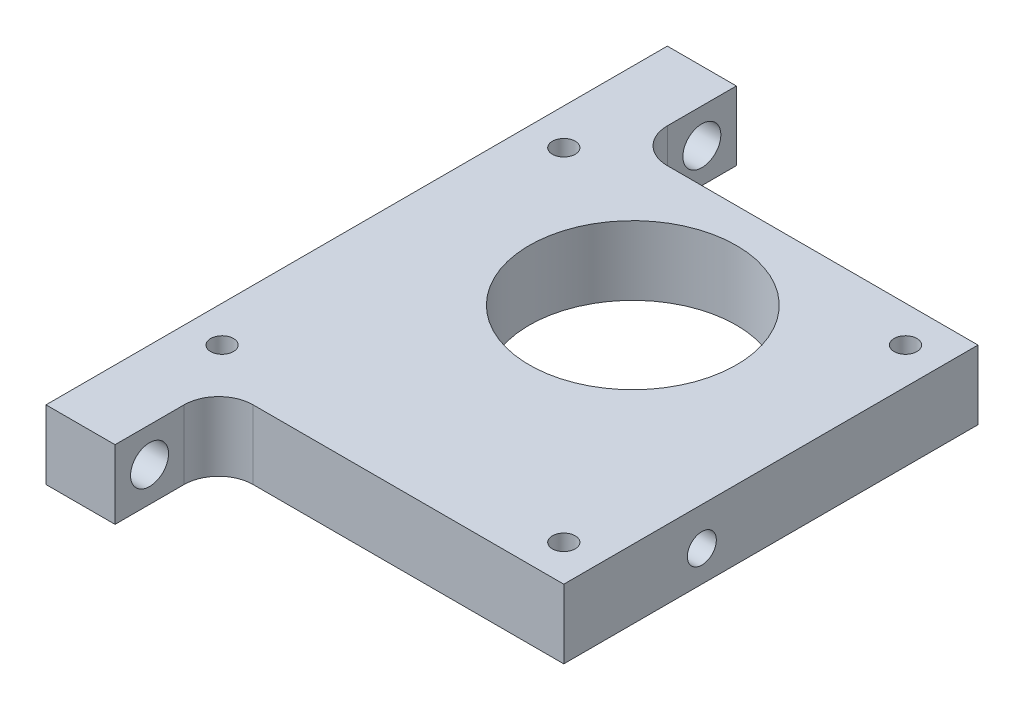
SolidWorks part; units mm, degrees
ref_plane "Front Plane" through (0, 0, 0) normal (0, 0, 1) x (1, 0, 0)
ref_plane "Top Plane" through (0, 0, 0) normal (0, 1, 0) x (1, 0, 0)
ref_plane "Right Plane" through (0, 0, 0) normal (1, 0, 0) x (0, 0, -1)
sketch "Sketch1" plane through (0, 0, 0) normal (0, 1, 0) x (1, 0, 0)
  line L1 (30, -45) -> (-30, -45)
  line L2 (30, -45) -> (30, 45)
  line L3 (30, 45) -> (-30, 45)
  line L4 (-30, -45) -> (-30, 45)
  line L5 (30, -45) -> (-30, 45) construction
  line L6 (30, 45) -> (-30, -45) construction
  point P0 (0, 0)
  dimension "D1" = 90
  dimension "D2" = 60
extrude "Boss-Extrude1" add sketch "Sketch1" along normal blind 10
sketch "Sketch4" plane through (0, 0, 0) normal (0, -1, 0) x (1, 0, 0)
  line L1 (0, 0) -> (0, -10) construction
  line L2 (30, -45) -> (-30, -45) construction
  circle A0 centre (0, -10) radius 15
  dimension "D1" = 35
  dimension "D2" = 30
extrude "Cut-Extrude3" cut sketch "Sketch4" against normal through all
hole_wizard "M4 Tapped Hole1" positions "Sketch6" profile "Sketch5" tap size "M4" standard "GB" end condition through all
sketch "Sketch6" plane through (0, 0, 0) normal (0, 1, 0) x (1, 0, 0)
  line L0 (-24.7487, -24.7475) -> (24.7487, -24.7475) construction
  line L1 (24.7487, -24.7475) -> (24.7487, 24.75) construction
  line L2 (24.7487, 24.75) -> (-24.7487, 24.75) construction
  line L3 (-24.7487, 24.75) -> (-24.7487, -24.7475) construction
  line L5 (0, 10) -> (0, 24.75) construction
  line L7 (0, 0) -> (0, 10) construction
  circle A0 centre (0, 0) radius 35 construction
  point P0 (-24.7487, -24.7475)
  point P3 (-24.7487, 24.75)
  point P6 (24.7487, 24.75)
  point P9 (24.7487, -24.7475)
  dimension "D4" = 70
  dimension "D1" = 49.4975
  dimension "D2" = 49.4975
  dimension "D3" = 14.75
  dimension "D5" = 10
sketch "Sketch5" plane through (-24.7487, 0, 24.7475) normal (1, 0, 0) x (0, 0, -1)
  line L0 (0, 0) -> (0, 10)
  line L1 (0, 10) -> (1.65, 10)
  line L2 (1.65, 10) -> (1.65, 0)
  line L5 (1.65, 0) -> (0, 0)
  line L11 (0, -6.35) -> (0, 107.95) construction
  dimension "通孔螺纹孔钻头直径" = 3.3
  dimension "通孔螺纹孔钻头深度" = 10
cosmetic thread "Cosmetic Thread12" parameters "D2"=4
cosmetic thread "Cosmetic Thread13" parameters "D2"=4
cosmetic thread "Cosmetic Thread14" parameters "D2"=4
cosmetic thread "Cosmetic Thread15" parameters "D2"=4
sketch "Sketch8" plane through (0, 0, 0) normal (0, -1, 0) x (1, 0, 0)
  line L0 (-20, 30) -> (-20, -30) construction
  line L1 (30, 45) -> (-20, 45)
  line L2 (30, 45) -> (30, 30)
  line L3 (30, 30) -> (-20, 30)
  line L4 (-20, 45) -> (-20, 30)
  line L5 (30, -45) -> (-20, -45)
  line L6 (30, -45) -> (30, -30)
  line L7 (30, -30) -> (-20, -30)
  line L8 (-20, -45) -> (-20, -30)
  line L9 (0, 0) -> (-20, 0) construction
  line L10 (-30, -45) -> (-30, 45) construction
  dimension "D1" = 10
  dimension "D2" = 15
extrude "Cut-Extrude5" cut sketch "Sketch8" against normal through all
other "Move Face1" [suppressed] parameters "D1"=10
hole_wizard "Ø5.5 (5.5) Diameter Hole1" positions "Sketch11" profile "Sketch10" hole size "Ø5.5" standard "GB"
sketch "Sketch11" plane through (-30, 0, 0) normal (-1, 0, 0) x (0, 0, 1)
  line L0 (-40, 5) -> (40, 5) construction
  line L2 (0, 0) -> (0, 5) construction
  line L3 (-45, 0) -> (45, 0) construction
  line L5 (-40, 5) -> (-45, 5) construction
  line L6 (-45, 10) -> (-45, 0) construction
  point P0 (-40, 5)
  point P2 (40, 5)
  dimension "D1" = 5
sketch "Sketch10" plane through (-30, 5, -40) normal (0, 1, 0) x (0, 0, 1)
  line L0 (0, 0) -> (0, 14.0524)
  line L1 (0, 14.0524) -> (2.75, 12.4)
  line L2 (2.75, 12.4) -> (2.75, 0)
  line L5 (2.75, 0) -> (0, 0)
  line L10 (0, 14.0524) -> (-2.75, 12.4) construction
  line L11 (0, -6.35) -> (0, 107.95) construction
  dimension "孔直径" = 5.5
  dimension "孔深度" = 12.4
  dimension "导头角度" = 118
fillet "Fillet1" radius 5 2 edges at (-20, 5, 30) (-20, 5, -30)
hole_wizard "M5 Tapped Hole1" positions "Sketch12" profile "Sketch13" tap size "M5" standard "GB"
sketch "Sketch12" plane through (30, 0, 0) normal (1, 0, 0) x (0, 0, -1)
  point P0 (-10.001, 4.5)
sketch "Sketch13" plane through (30, 4.5, 10.001) normal (0, 1, 0) x (0, 0, -1)
  line L0 (0, 0) -> (0, 13.6618)
  line L1 (0, 13.6618) -> (2.1, 12.4)
  line L2 (2.1, 12.4) -> (2.1, 0)
  line L5 (2.1, 0) -> (0, 0)
  line L10 (0, 13.6618) -> (-2.1, 12.4) construction
  line L11 (0, -6.35) -> (0, 107.95) construction
  dimension "螺纹孔钻头直径" = 4.2
  dimension "螺纹孔钻头深度" = 12.4
  dimension "导头角度" = 118
cosmetic thread "Cosmetic Thread16" parameters "D1"=10, "D2"=5
